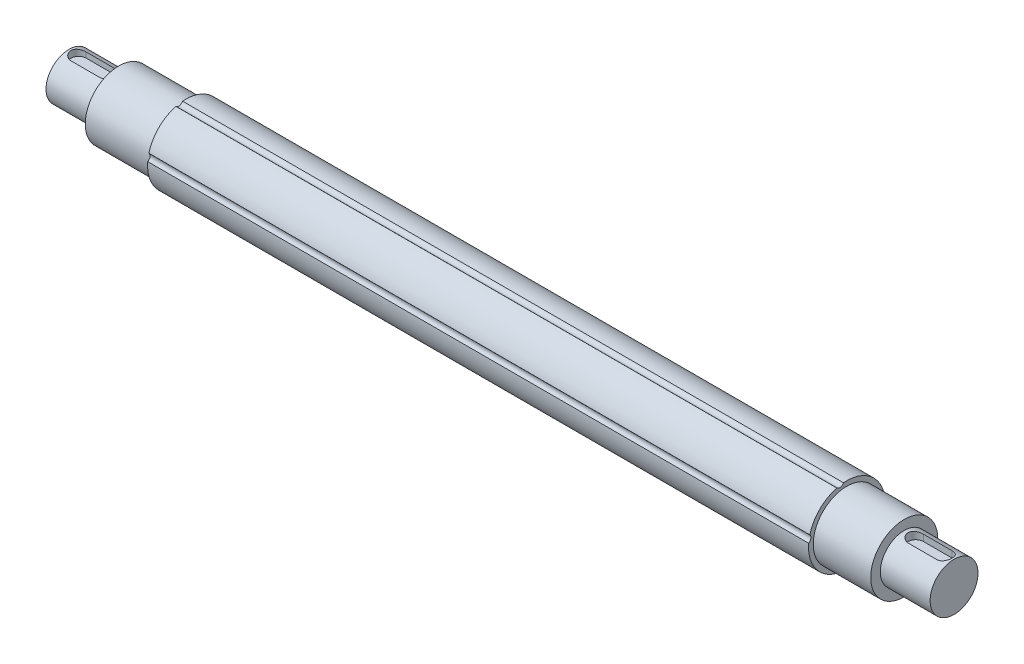
from build123d import *

# Parameters (mm, degrees)
CUT_EXTRUDE_1_DEPTH      = 205.5
CUT_EXTRUDE_1_DEPTH_BACK = 205.5
SKETCH_2_R               = 40
SKETCH_3_OUTSIDE_W       = 124.974
SKETCH_3_OUTSIDE_H       = 124.974
SKETCH_3_OUTSIDE_R       = 17.5
CUT_EXTRUDE_2_DEPTH      = 18
SKETCH_4_OUTSIDE_W       = 124.974
SKETCH_4_OUTSIDE_H       = 124.974
SKETCH_4_OUTSIDE_R       = 12.5
CUT_EXTRUDE_3_DEPTH      = 26
SKETCH_5_OUTSIDE_W       = 124.974
SKETCH_5_OUTSIDE_H       = 124.974
SKETCH_5_OUTSIDE_R       = 17.5
CUT_EXTRUDE_4_DEPTH      = 30
CUT_EXTRUDE_5_DEPTH      = 4
SKETCH_7_R               = 17.5
EXTRUDE_1_DEPTH          = 51
SKETCH_9_OUTSIDE_W       = 135.09
SKETCH_9_OUTSIDE_H       = 135.09
SKETCH_9_OUTSIDE_R       = 12
CUT_EXTRUDE_7_DEPTH      = 26
MOVE_FACE_1_BY           = 8


with BuildPart() as part:
    # 草图1 → 旋转1 (revolve)
    with BuildSketch(Plane.XY, mode=Mode.PRIVATE) as revolve_1_sk:
        Polygon((-205.5, 0), (-205.5, 19), (-204.5, 20), (204.5, 20), (205.5, 19), (205.5, 0), align=None)
    revolve(revolve_1_sk.sketch.rotate(Axis((205.5, 0, 0), (-1, 0, 0)), 270), axis=Axis((205.5, 0, 0), (-1, 0, 0)))

    # 草图2 → 切除-拉伸1 (cut, two sides: drawn at the far end of the back side and taken through both)
    with BuildSketch(Plane(origin=(0, 0, 0), x_dir=(0, 0, -1), z_dir=(1, 0, 0)).offset(-CUT_EXTRUDE_1_DEPTH_BACK)):
        Circle(SKETCH_2_R)
        with BuildLine():
            ThreePointArc((-19.926297295, 1.715423015), (-14.142135624, -14.142135624), (1.715423015, -19.926297295))
            ThreePointArc((1.715423015, -19.926297295), (3.302788339, -18.731043462), (5.203224708, -19.311303753))
            ThreePointArc((5.203224708, -19.311303753), (14.142135624, -14.142135624), (19.311303753, -5.203224708))
            ThreePointArc((19.311303753, -5.203224708), (18.731043462, -3.302788339), (19.926297295, -1.715423015))
            ThreePointArc((19.926297295, -1.715423015), (14.142135624, 14.142135624), (-1.715423015, 19.926297295))
            ThreePointArc((-1.715423015, 19.926297295), (-3.302788339, 18.731043462), (-5.203224708, 19.311303753))
            ThreePointArc((-5.203224708, 19.311303753), (-14.142135624, 14.142135624), (-19.311303753, 5.203224708))
            ThreePointArc((-19.311303753, 5.203224708), (-18.731043462, 3.302788339), (-19.926297295, 1.715423015))
        make_face(mode=Mode.SUBTRACT)
    extrude(amount=CUT_EXTRUDE_1_DEPTH + CUT_EXTRUDE_1_DEPTH_BACK, mode=Mode.SUBTRACT)

    # 草图3 outside → 切除-拉伸2 (cut)
    with BuildSketch(Plane.ZY.offset(205.5)):
        Rectangle(SKETCH_3_OUTSIDE_W, SKETCH_3_OUTSIDE_H)
        Circle(SKETCH_3_OUTSIDE_R, mode=Mode.SUBTRACT)
    extrude(amount=-CUT_EXTRUDE_2_DEPTH, mode=Mode.SUBTRACT)

    # 草图4 outside → 切除-拉伸3 (cut)
    with BuildSketch(Plane(origin=(205.5, 0, 0), x_dir=(0, 0, -1), z_dir=(1, 0, 0))):
        Rectangle(SKETCH_4_OUTSIDE_W, SKETCH_4_OUTSIDE_H)
        Circle(SKETCH_4_OUTSIDE_R, mode=Mode.SUBTRACT)
    extrude(amount=-CUT_EXTRUDE_3_DEPTH, mode=Mode.SUBTRACT)

    # 草图5 outside → 切除-拉伸4 (cut)
    with BuildSketch(Plane(origin=(179.5, 0, 0), x_dir=(0, 0, -1), z_dir=(1, 0, 0))):
        Rectangle(SKETCH_5_OUTSIDE_W, SKETCH_5_OUTSIDE_H)
        with Locations(Location((0, 0, 0), (0, 0, 180))):
            Circle(SKETCH_5_OUTSIDE_R, mode=Mode.SUBTRACT)
    extrude(amount=-CUT_EXTRUDE_4_DEPTH, mode=Mode.SUBTRACT)

    # 草图6 → 切除-拉伸5 (cut)
    with BuildSketch(Plane(origin=(0, 12.5, 0), x_dir=(1, 0, 0), z_dir=(0, 1, 0))):
        with BuildLine():
            Line((200.5, -4), (185.5, -4))
            ThreePointArc((185.5, -4), (181.5, 0), (185.5, 4))
            Line((185.5, 4), (200.5, 4))
            ThreePointArc((200.5, 4), (204.5, 0), (200.5, -4))
        make_face()
    cut_extrude_5 = extrude(amount=-CUT_EXTRUDE_5_DEPTH, mode=Mode.SUBTRACT)

    # 草图7 → 凸台-拉伸1 (add)
    with BuildSketch(Plane.ZY.offset(205.5)):
        Circle(SKETCH_7_R)
    extrude(amount=EXTRUDE_1_DEPTH)

    # 草图9 outside → 切除-拉伸7 (cut)
    with BuildSketch(Plane.ZY.offset(256.5)):
        Rectangle(SKETCH_9_OUTSIDE_W, SKETCH_9_OUTSIDE_H)
        Circle(SKETCH_9_OUTSIDE_R, mode=Mode.SUBTRACT)
    extrude(amount=-CUT_EXTRUDE_7_DEPTH, mode=Mode.SUBTRACT)

    # 镜向1: 切除-拉伸5 across plane
    add(cut_extrude_5.mirror(Plane.ZY.offset(25.5)), mode=Mode.SUBTRACT)

    # Move Face 1: a face moved outward by 8.0
    extrude(part.faces().sort_by_distance((-187.5, -16, -10))[0], amount=MOVE_FACE_1_BY, dir=(-1, 0, 0))


solid = part.part
